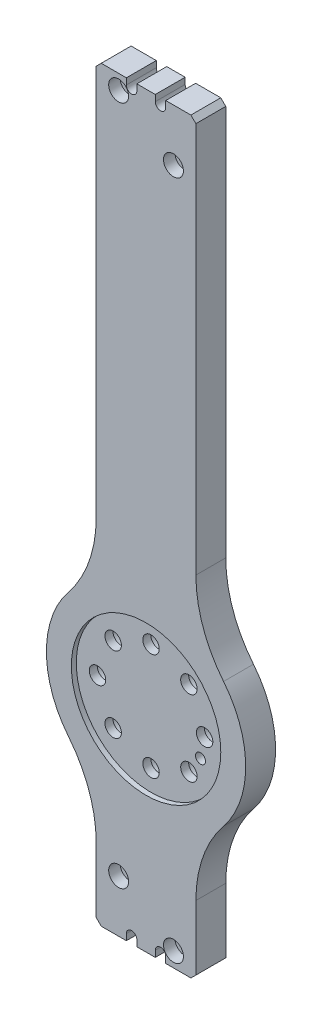
SolidWorks part; units mm, degrees
ref_plane "前视基准面" through (0, 0, 0) normal (0, 0, 1) x (1, 0, 0)
ref_plane "上视基准面" through (0, 0, 0) normal (0, 1, 0) x (1, 0, 0)
ref_plane "右视基准面" through (0, 0, 0) normal (1, 0, 0) x (0, 0, -1)
sketch "草图1" plane through (0, 0, 0) normal (0, 0, 1) x (1, 0, 0)
  line L1 (-40, -150) -> (40, -150)
  line L2 (-40, -150) -> (-40, 150)
  line L3 (-40, 150) -> (40, 150)
  line L4 (40, -150) -> (40, 150)
  line L5 (-40, -150) -> (40, 150) construction
  line L6 (-40, 150) -> (40, -150) construction
  point P0 (0, 0)
  dimension "D1" = 80
  dimension "D2" = 300
extrude "凸台-拉伸1" add sketch "草图1" along normal blind 12 contours L3 L4 L1 L2
chamfer "倒角1" distance 2 angle 45 4 edges at (-40, 150, 6) (40, 150, 6) (40, -150, 6) (-40, -150, 6)
sketch "草图2" plane through (0, 0, 12) normal (0, 0, 1) x (1, 0, 0)
  line L0 (-38, -150) -> (38, -150) construction
  circle A0 centre (0, -65.5) radius 30
  point P6 (0, -150)
  dimension "D1" = 60
  dimension "D2" = 65.5
extrude "切除-拉伸1" cut sketch "草图2" against normal blind 2
sketch "草图3" plane through (0, 0, 12) normal (0, 0, 1) x (1, 0, 0)
  line L0 (-20, -150) -> (-20, -100.141)
  line L1 (-38, -150) -> (38, -150) construction
  line L2 (0, 0) -> (0, -182.0537) construction
  line L5 (20, -150) -> (20, -100.141)
  line L6 (20, 150) -> (20, -30.859)
  line L7 (-20, 150) -> (-20, -30.859)
  line L8 (-20, 150) -> (-38, 150)
  line L9 (20, -150) -> (38, -150)
  line L16 (38, 150) -> (-38, 150)
  line L17 (-38, 150) -> (-40, 148)
  line L18 (-40, 148) -> (-40, -148)
  line L19 (-40, -148) -> (-38, -150)
  line L20 (-38, -150) -> (38, -150)
  line L21 (38, -150) -> (40, -148)
  line L22 (40, -148) -> (40, 148)
  line L23 (40, 148) -> (38, 150)
  line L24 (38, 150) -> (20, 150)
  line L25 (-38, 150) -> (-40, 148)
  line L26 (-40, 148) -> (-40, -148)
  line L27 (-40, -148) -> (-38, -150)
  line L28 (-38, -150) -> (-20, -150)
  line L29 (38, -150) -> (40, -148)
  line L30 (40, -148) -> (40, 148)
  line L31 (40, 148) -> (38, 150)
  arc A2 (20, -100.141) -> (20, -30.859) centre (0, -65.5) ccw
  circle A3 centre (0, -65.5) radius 40
  arc A4 (-20, -30.859) -> (-20, -100.141) centre (0, -65.5) ccw
  dimension "D1" = 20
  dimension "D4" = 40
  dimension "D2" = 0
  dimension "D3" = 10
extrude "切除-拉伸2" cut sketch "草图3" against normal through all
fillet "圆角1" radius 50 4 edges at (20, -100.141, 6) (20, -30.859, 6) (-20, -100.141, 6) (-20, -30.859, 6)
chamfer "倒角3" distance 2 angle 45 4 edges at (-20, 150, 6) (20, 150, 6) (-20, -150, 6) (20, -150, 6)
sketch "草图6" plane through (0, 0, 0) normal (0, 0, -1) x (-1, 0, 0)
  line L0 (0, 0) -> (-13.6308, 0) construction
  point P8 (0, -87)
hole_wizard "M6 六角圆柱头螺钉的柱形沉头孔1" positions "草图6" profile "草图7" counterbore size "M6" standard "GB" end condition through all
sketch "草图7" plane through (0, -87, 0) normal (1, 0, 0) x (0, 1, 0)
  line L0 (0, 0) -> (0, 12)
  line L1 (0, 12) -> (3.3, 12)
  line L3 (3.3, 12) -> (3.3, 6.8)
  line L4 (3.3, 6.8) -> (5.5, 6.8)
  line L5 (5.5, 6.8) -> (5.5, 0)
  line L7 (5.5, 0) -> (0, 0)
  line L11 (0, -6.35) -> (0, 107.95) construction
  dimension "通孔孔直径" = 6.6
  dimension "通孔孔深度" = 12
  dimension "柱形沉头孔直径" = 11
  dimension "柱形沉头孔深度" = 6.8
sketch "草图10" plane through (0, 0, 0) normal (0, 0, -1) x (-1, 0, 0)
  line L2 (0, 0) -> (-18.9395, -7.845) construction
  line L3 (0, -65.5) -> (-70.8488, -94.8465) construction
  line L5 (0, -65.5) -> (53.714, -65.5) construction
  circle A0 centre (0, -65.5) radius 21.5 construction
  point P0 (-19.8634, -73.7277)
  dimension "D2" = 43
  dimension "D1" = 22.5
hole_wizard "Ø4.0mm 暗销孔1" positions "草图10" profile "草图9" hole size "Ø4.0" standard "GB" end condition through all
sketch "草图9" plane through (19.8634, -73.7277, 0) normal (1, 0, 0) x (0, 1, 0)
  line L0 (0, 0) -> (0, 12)
  line L1 (0, 12) -> (2, 12)
  line L2 (2, 12) -> (2, 0)
  line L5 (2, 0) -> (0, 0)
  line L11 (0, -6.35) -> (0, 107.95) construction
  dimension "通孔孔直径" = 4
  dimension "通孔孔深度" = 12
sketch "草图13" plane through (0, 0, 12) normal (0, 0, 1) x (1, 0, 0)
  line L0 (0, 0) -> (76.9365, 0) construction
  point P0 (-11, -129.05)
  point P3 (11, -144.05)
  point P12 (-11, 144.05)
  point P13 (11, 129.05)
hole_wizard "M4 六角圆柱头螺钉的柱形沉头孔1" positions "草图13" profile "草图12" counterbore size "M4" standard "GB" end condition through all
sketch "草图12" plane through (-11, -129.05, 12) normal (1, 0, 0) x (0, -1, 0)
  line L0 (0, 0) -> (0, 12)
  line L1 (0, 12) -> (2.25, 12)
  line L3 (2.25, 12) -> (2.25, 4.6)
  line L4 (2.25, 4.6) -> (4, 4.6)
  line L5 (4, 4.6) -> (4, 0)
  line L7 (4, 0) -> (0, 0)
  line L11 (0, -6.35) -> (0, 107.95) construction
  dimension "通孔孔直径" = 4.5
  dimension "通孔孔深度" = 12
  dimension "柱形沉头孔直径" = 8
  dimension "柱形沉头孔深度" = 4.6
sketch "草图14" plane through (0, 0, 12) normal (0, 0, 1) x (1, 0, 0)
  line L0 (5.8, -147.5) -> (5.8, -150) construction
  line L1 (-18, -150) -> (18, -150) construction
  line L2 (7.9, -147.5) -> (7.9, -150)
  line L3 (3.7, -147.5) -> (3.7, -150)
  line L4 (-5.8, -147.5) -> (-5.8, -150) construction
  line L5 (-3.7, -147.5) -> (-3.7, -150)
  line L6 (-7.9, -147.5) -> (-7.9, -150)
  line L7 (0, 0) -> (56.1675, 0) construction
  line L8 (5.8, 147.5) -> (5.8, 150) construction
  line L9 (7.9, 147.5) -> (7.9, 150)
  line L10 (3.7, 147.5) -> (3.7, 150)
  line L11 (-5.8, 147.5) -> (-5.8, 150) construction
  line L12 (-3.7, 147.5) -> (-3.7, 150)
  line L13 (-7.9, 147.5) -> (-7.9, 150)
  arc A0 (7.9, -147.5) -> (3.7, -147.5) centre (5.8, -147.5) ccw
  arc A1 (3.7, -150) -> (7.9, -150) centre (5.8, -150) ccw
  arc A2 (-3.7, -147.5) -> (-7.9, -147.5) centre (-5.8, -147.5) ccw
  arc A3 (-7.9, -150) -> (-3.7, -150) centre (-5.8, -150) ccw
  arc A4 (7.9, 147.5) -> (3.7, 147.5) centre (5.8, 147.5) cw
  arc A5 (3.7, 150) -> (7.9, 150) centre (5.8, 150) cw
  arc A6 (-3.7, 147.5) -> (-7.9, 147.5) centre (-5.8, 147.5) cw
  arc A7 (-7.9, 150) -> (-3.7, 150) centre (-5.8, 150) cw
  point P5 (5.8, -148.75)
  point P13 (-5.8, -148.75)
  point P24 (5.8, 148.75)
  point P31 (-5.8, 148.75)
  dimension "D1" = 2.1
  dimension "D2" = 2.1
  dimension "D3" = 2.5
  dimension "D4" = 2.5
extrude "切除-拉伸3" cut sketch "草图14" against normal through all
pattern_circular "阵列(圆周)1" count 8 over 360 about axis through (0, -65.5, 0) along (0, 0, 1) of "M6 六角圆柱头螺钉的柱形沉头孔1"
